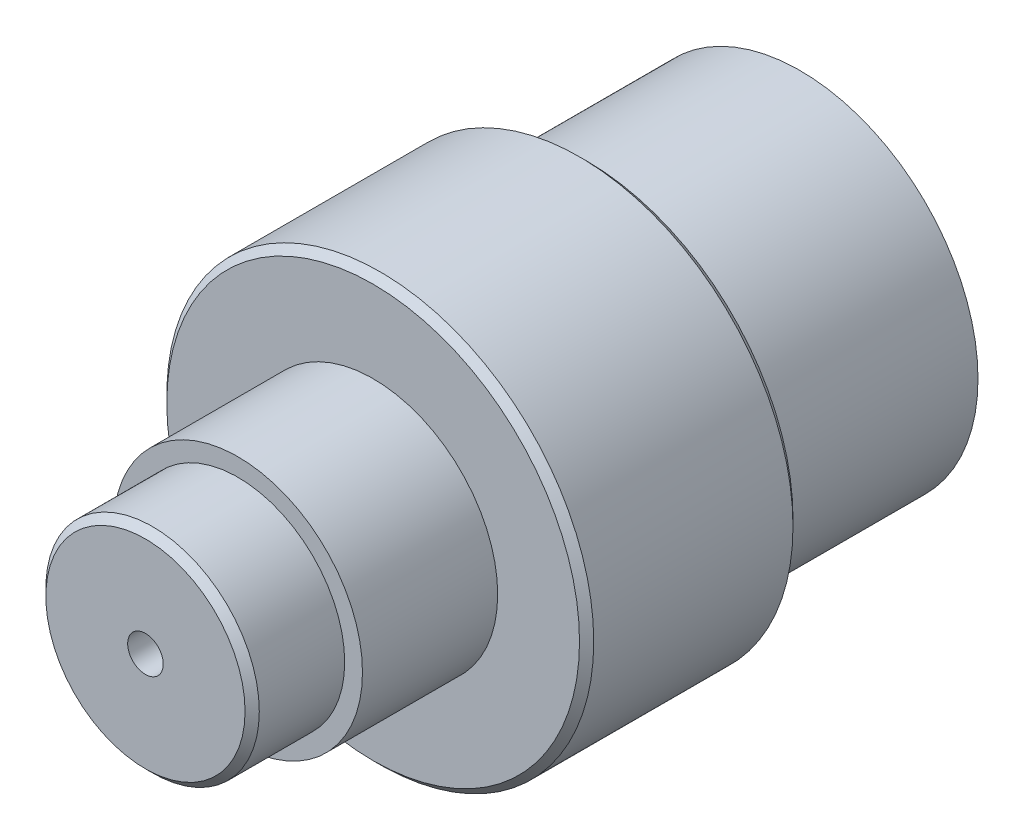
from build123d import *

# Parameters (mm, degrees)
SKETCH_1_R             = 25
EXTRUDE_1_DEPTH        = 30
SKETCH_2_R             = 30
EXTRUDE_2_DEPTH        = 30
SKETCH_4_R             = 15
CUT_EXTRUDE_1_DEPTH    = 74.484692283
EXTRUDE_START          = -30
SKETCH_13_R            = 15
EXTRUDE_4_DEPTH        = 30
SKETCH_12_R            = 17.5
EXTRUDE_3_DEPTH        = 32
HOLE_WIZARD_M6_1_D     = 5
HOLE_WIZARD_M6_1_DEPTH = 15
HOLE_WIZARD_M6_1_TIP   = 1.502151548
CUT_EXTRUDE_START      = -13
SKETCH_16_R            = 17.5
SKETCH_16_R_2          = 15
CUT_EXTRUDE_3_DEPTH    = 13
CHAMFER_4_SIZE         = 1


with BuildPart() as part:
    # 草图1 → 凸台-拉伸1 (new body)
    with BuildSketch(Plane.XY):
        Circle(SKETCH_1_R)
    extrude(amount=EXTRUDE_1_DEPTH)

    # 草图2 → 凸台-拉伸2 (add)
    with BuildSketch(Plane.XY.offset(30)):
        Circle(SKETCH_2_R)
    extrude(amount=EXTRUDE_2_DEPTH)

    # 草图4 → 切除-拉伸1 (cut, through all)
    with BuildSketch(Plane(origin=(0, 0, 0), x_dir=(-1, 0, 0), z_dir=(0, 0, -1))):
        Circle(SKETCH_4_R)
    extrude(amount=-CUT_EXTRUDE_1_DEPTH, mode=Mode.SUBTRACT)

    # 草图13 → 凸台-拉伸4 (add)
    with BuildSketch(Plane.XY.offset(60).offset(EXTRUDE_START)):
        with Locations(Location((0, 0, 0), (0, 0, 180))):
            Circle(SKETCH_13_R)
    extrude(amount=EXTRUDE_4_DEPTH)

    # 草图12 → 凸台-拉伸3 (add)
    with BuildSketch(Plane.XY.offset(60)):
        Circle(SKETCH_12_R)
    extrude(amount=EXTRUDE_3_DEPTH)

    # M6 螺纹孔1
    with Locations(Plane.XY.offset(92)):
        with Locations((0, 0)):
            Hole(HOLE_WIZARD_M6_1_D / 2, depth=HOLE_WIZARD_M6_1_DEPTH)
            with Locations((0, 0, -(HOLE_WIZARD_M6_1_DEPTH + HOLE_WIZARD_M6_1_TIP / 2))):  # 118° drill point
                Cone(0, HOLE_WIZARD_M6_1_D / 2, HOLE_WIZARD_M6_1_TIP, mode=Mode.SUBTRACT)

    # 草图16 → 切除-拉伸3 (cut)
    with BuildSketch(Plane.XY.offset(92).offset(CUT_EXTRUDE_START)):
        Circle(SKETCH_16_R)
        with Locations(Location((0, 0, 0), (0, 0, 180))):
            Circle(SKETCH_16_R_2, mode=Mode.SUBTRACT)
    extrude(amount=CUT_EXTRUDE_3_DEPTH, mode=Mode.SUBTRACT)

    # 倒角4
    chamfer_4_edges = [part.edges().sort_by_distance(p)[0] for p in [
        (15, 0, 0),
        (15, 0, 92),
        (-30, 0, 30),
        (-30, 0, 60),
    ]]
    chamfer(chamfer_4_edges, length=CHAMFER_4_SIZE)


solid = part.part
